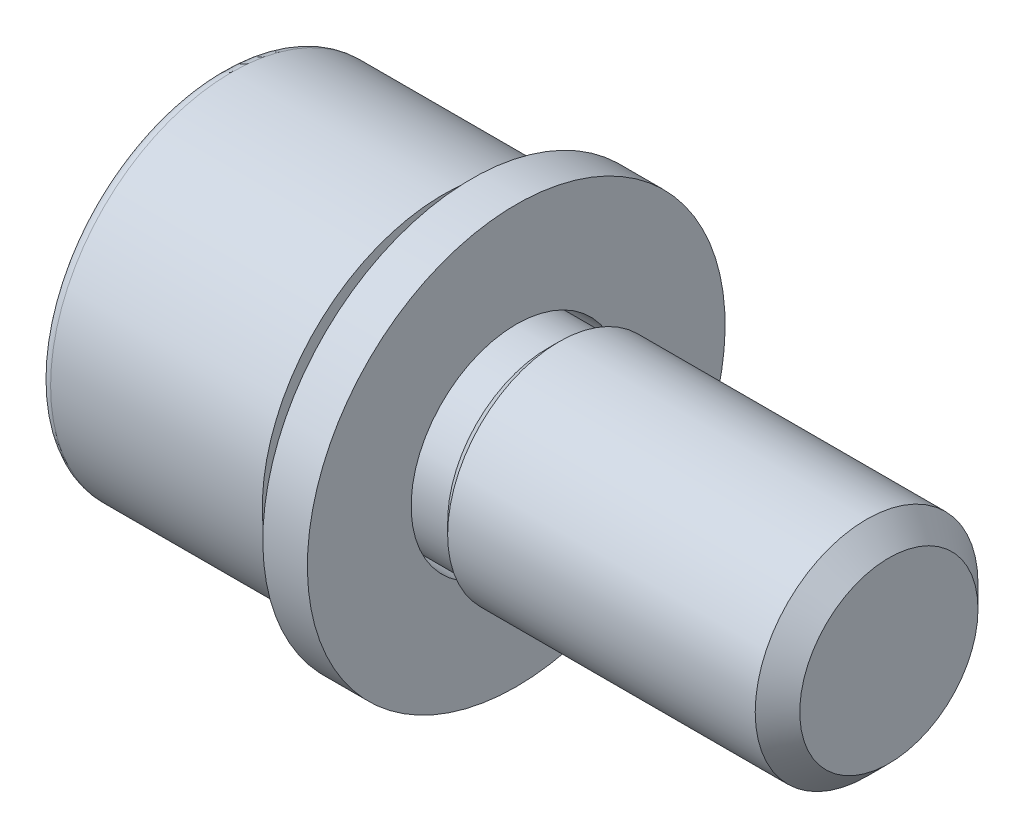
SolidWorks part; units mm, degrees
ref_plane "Front Plane" through (0, 0, 0) normal (0, 0, 1) x (1, 0, 0)
ref_plane "Top Plane" through (0, 0, 0) normal (0, 1, 0) x (1, 0, 0)
ref_plane "Right Plane" through (0, 0, 0) normal (1, 0, 0) x (0, 0, -1)
sketch "Dimension Sketch" plane through (0, 0, 0) normal (0, 0, 1) x (1, 0, 0)
  line L0 (0, 0) -> (24, 0) construction
  point P2 (9.2, 0)
  point P3 (17.14, 0)
  point P4 (22.75, 0)
  point P5 (4, 0)
  point P6 (13, 0)
  point P7 (8, 0)
  point P8 (8, 0)
  point P9 (20.188, 0)
  point P10 (21.208, 0)
  point P11 (0.4, 0)
  point P12 (-4, 0)
  point P14 (11.14, 0)
  point P15 (22.008, 0)
  point P16 (0, 12.33)
  point P17 (0, 9.03)
  dimension "k" = 8
  dimension "l" = 16
  dimension "t" = 4
  dimension "dk" = 13
  dimension "d" = 8
  dimension "da" = 9.2
  dimension "b" = 28
  dimension "e" = 6.86
  dimension "p" = 1.25
  dimension "ds" = 7.188
  dimension "lf" = 1.02
  dimension "r" = 0.4
  dimension "s" = 6
  dimension "v" = 0.8
  dimension "dw" = 12.33
  dimension "w" = 3.3
sketch "Sketch1" plane through (0, 0, 0) normal (0, 0, 1) x (1, 0, 0)
  line L1 (0, 0) -> (0, 6.5)
  line L2 (0, 6.5) -> (8, 6.5)
  line L3 (8, 6.5) -> (8, 4.6)
  line L4 (9.02, 3.594) -> (11.75, 3.594)
  line L5 (24, 4) -> (24, 0)
  line L6 (0, 0) -> (24, 0)
  line L7 (0, 0) -> (-33.993, 0) construction
  line L8 (8.1204, 4.3139) -> (8.7404, 3.7079)
  line L9 (11.75, 3.594) -> (12.156, 4)
  line L10 (12.156, 4) -> (24, 4)
  line L11 (6.6803, 0) -> (4.7, 3.43) construction
  line L12 (4.7, 3.43) -> (0, 3.43) construction
  line L13 (6.6803, 0) -> (4.7, -3.43) construction
  line L14 (4.7, -3.43) -> (0, -3.43) construction
  arc A0 (9.02, 3.594) -> (8.7404, 3.7079) centre (9.02, 3.994) cw
  arc A1 (8.1204, 4.3139) -> (8, 4.6) centre (8.4, 4.6) cw
  point P10 (4.7, 6.5)
  point P21 (0.634, 6.5)
  dimension "D1" = 0.4
  dimension "D2" = 8
  dimension "dk" = 13
  dimension "D3" = 8
  dimension "l" = 16
  dimension "D5" = 45
  dimension "da" = 9.2
  dimension "lt" = 1.02
  dimension "ds" = 7.188
  dimension "ls" = 3.75
  dimension "D6" = 120
  dimension "w" = 3.3
  dimension "D7" = 6.86
  dimension "f" = 0.634
revolve "Base-Revolve" add sketch "Sketch1" angle 360 about L7
cosmetic thread "Cosmetic Thread1" parameters "D1"=12.25, "D2"=6.6469
sketch "Sketch2" plane through (0, 0, 0) normal (-1, 0, 0) x (0, 0, 1)
  line L1 (2.9705, -1.715) -> (2.9705, 1.715)
  line L2 (2.9705, 1.715) -> (0, 3.43)
  line L3 (0, 3.43) -> (-2.9705, 1.715)
  line L4 (-2.9705, 1.715) -> (-2.9705, -1.715)
  line L5 (-2.9705, -1.715) -> (0, -3.43)
  line L6 (0, -3.43) -> (2.9705, -1.715)
  circle A0 centre (0, 0) radius 2.9705 construction
  dimension "e" = 6.86
extrude "Cut-Extrude1" cut sketch "Sketch2" against normal up to vertex (4.7 mm away) up to point (4.7, 3.43, 0)
ref_plane "Plane1" through (6.6803, 0, 0) normal (1, 0, 0) x (0, 0, -1)
sketch "Sketch13" plane through (0, 0, 0) normal (0, 0, 1) x (1, 0, 0)
  line L0 (0, 3.43) -> (0.4595, 2.9705)
  line L1 (0.4595, 2.9705) -> (0, 2.9705)
  line L2 (0, 0) -> (0, 6.5) construction
  line L3 (0, 2.9705) -> (0, 3.43)
  line L6 (0, 0) -> (-33.993, 0) construction
  line L7 (0, 0) -> (-33.993, 0) construction
  line L8 (4.7, 3.43) -> (0, 3.43) construction
  line L9 (4.7, 3.43) -> (0, 3.43) construction
  line L10 (2.35, 3.43) -> (2.35, 0) construction
  line L11 (0, 0) -> (24, 0) construction
  line L12 (4.7, 2.9705) -> (4.7, 3.43) construction
  line L13 (4.2405, 2.9705) -> (4.7, 2.9705) construction
  line L14 (4.7, 3.43) -> (4.2405, 2.9705) construction
  dimension "D1" = 45
revolve "Cut-Revolve4" cut sketch "Sketch13" angle 360 mid plane about L7
sketch "Sketch16" plane through (0, 0, 0) normal (0, 0, 1) x (1, 0, 0)
  line L0 (6.6803, 0) -> (4.7, 3.43) construction
  line L1 (0, 0) -> (24, 0) construction
  line L2 (6.6803, 0) -> (4.7, 3.43)
  line L3 (4.7, 0) -> (6.6803, 0)
  line L4 (4.7, 3.43) -> (4.7, 0)
revolve "Cut-Revolve5" cut sketch "Sketch16" angle 360 mid plane about L3
fillet "Fillet1" radius 0.4 1 edges at (0, 0, -6.5)
sketch "Sketch11" plane through (0, 0, 0) normal (0, 0, 1) x (1, 0, 0)
  line L0 (9.02, 3.775) -> (9.02, 7.5)
  line L1 (9.02, 7.5) -> (10.62, 7.5)
  line L2 (10.62, 7.5) -> (10.62, 3.775)
  line L3 (10.62, 3.775) -> (9.02, 3.775)
  line L4 (0, 0) -> (24, 0) construction
  line L5 (0, 0) -> (24, 0) construction
  dimension "垫圈d" = 7.55
  dimension "h" = 1.6
  dimension "d2" = 15
revolve "Revolve1" add sketch "Sketch11" angle 360 mid plane about L5
chamfer "Chamfer1" distance 0.8 angle 45 1 edges at (24, 0, -4)
